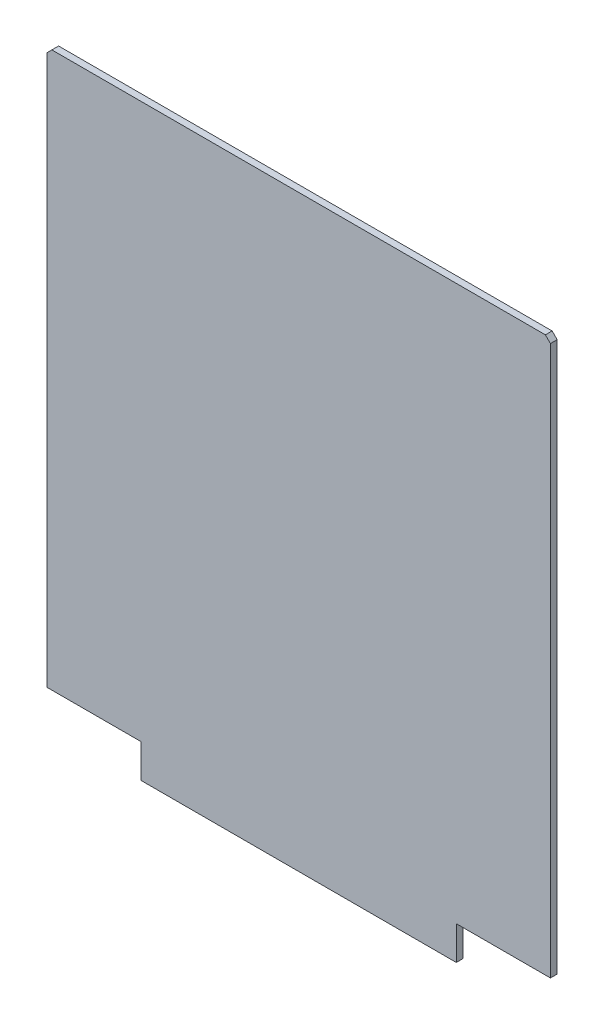
from build123d import *

# Parameters (mm, degrees)
EXTRUDE_1_DEPTH = 16
CHAMFER_1_SIZE  = 12


with BuildPart() as part:
    # 草图1 → 凸台-拉伸1 (new body)
    with BuildSketch(Plane.XY):
        Polygon((-599, -819), (-375, -819), (-375, -899), (375, -899), (375, -819), (599, -819), (599, 500), (-599, 500), align=None)
    extrude(amount=EXTRUDE_1_DEPTH)

    # 倒角1
    chamfer_1_edges = [part.edges().sort_by_distance(p)[0] for p in [
        (-599, 500, 8),
        (599, 500, 8),
    ]]
    chamfer(chamfer_1_edges, length=CHAMFER_1_SIZE)


solid = part.part
